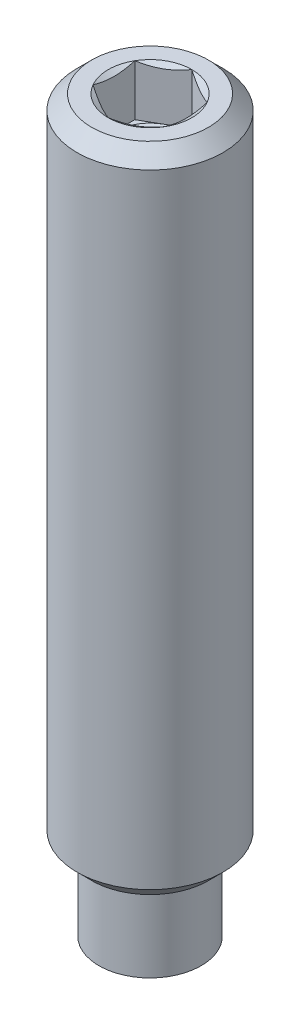
SolidWorks part; units mm, degrees
material "45"
ref_plane "Front Plane" through (0, 0, 0) normal (0, 0, 1) x (1, 0, 0)
ref_plane "Top Plane" through (0, 0, 0) normal (0, 1, 0) x (1, 0, 0)
ref_plane "Right Plane" through (0, 0, 0) normal (1, 0, 0) x (0, 0, -1)
sketch "Sketch1" plane through (0, 0, 0) normal (0, 1, 0) x (1, 0, 0)
  circle A0 centre (0, 0) radius 5
  dimension "D1" = 10
extrude "Boss-Extrude1" add sketch "Sketch1" along normal blind 15
sketch "Sketch2" plane through (0, 0, 0) normal (0, -1, 0) x (1, 0, 0)
  circle A0 centre (0, 0) radius 5
  dimension "D1" = 10
extrude "Boss-Extrude2" add sketch "Sketch2" along normal blind 35
cosmetic thread "Cosmetic Thread1" parameters "D2"=8.376
sketch "Sketch3" plane through (0, 15, 0) normal (0, 1, 0) x (1, 0, 0)
  line L1 (0, 2.8615) -> (-2.4781, 1.4307)
  line L2 (-2.4781, 1.4307) -> (-2.4781, -1.4308)
  line L3 (-2.4781, -1.4308) -> (0, -2.8615)
  line L4 (0, -2.8615) -> (2.4781, -1.4308)
  line L5 (2.4781, -1.4308) -> (2.4781, 1.4308)
  line L6 (2.4781, 1.4308) -> (0, 2.8615)
  circle A0 centre (0, 0) radius 2.8615 construction
  dimension "D1" = 5.723
extrude "Cut-Extrude1" cut sketch "Sketch3" against normal blind 3.5
sketch "Sketch4" plane through (0, 0, 0) normal (0, 0, 1) x (1, 0, 0)
  line L0 (0, 11.5) -> (2.4781, 11.5) construction
  line L1 (2.4781, 11.5) -> (2.4781, 15) construction
  line L2 (5, 15) -> (-5, 15) construction
  line L3 (0, 11.5) -> (2.4781, 11.5)
  line L4 (2.4781, 14.7787) -> (2.4781, 15)
  line L5 (2.8615, 15) -> (2.4781, 15)
  line L6 (0, -3.9322) -> (0, 17.1112) construction
  line L7 (2.4781, 11.5) -> (0, 10.0692)
  line L8 (0, 10.0692) -> (0, 11.5)
  line L9 (2.8615, 15) -> (2.4781, 14.7787)
  dimension "D1" = 60
  dimension "D2" = 5.723
  dimension "D3" = 60
revolve "Cut-Revolve1" cut sketch "Sketch4" angle 360 about L6
sketch "Sketch5" plane through (0, -35, 0) normal (0, -1, 0) x (1, 0, 0)
  circle A0 centre (0, 0) radius 5 construction
  circle A1 centre (0, 0) radius 5
  circle A2 centre (0, 0) radius 3.5
  dimension "D1" = 7
extrude "Cut-Extrude2" cut sketch "Sketch5" against normal blind 5.3
chamfer "Chamfer1" distance 1 angle 45 2 edges at (0, -29.7, -5) (0, 15, 5)
